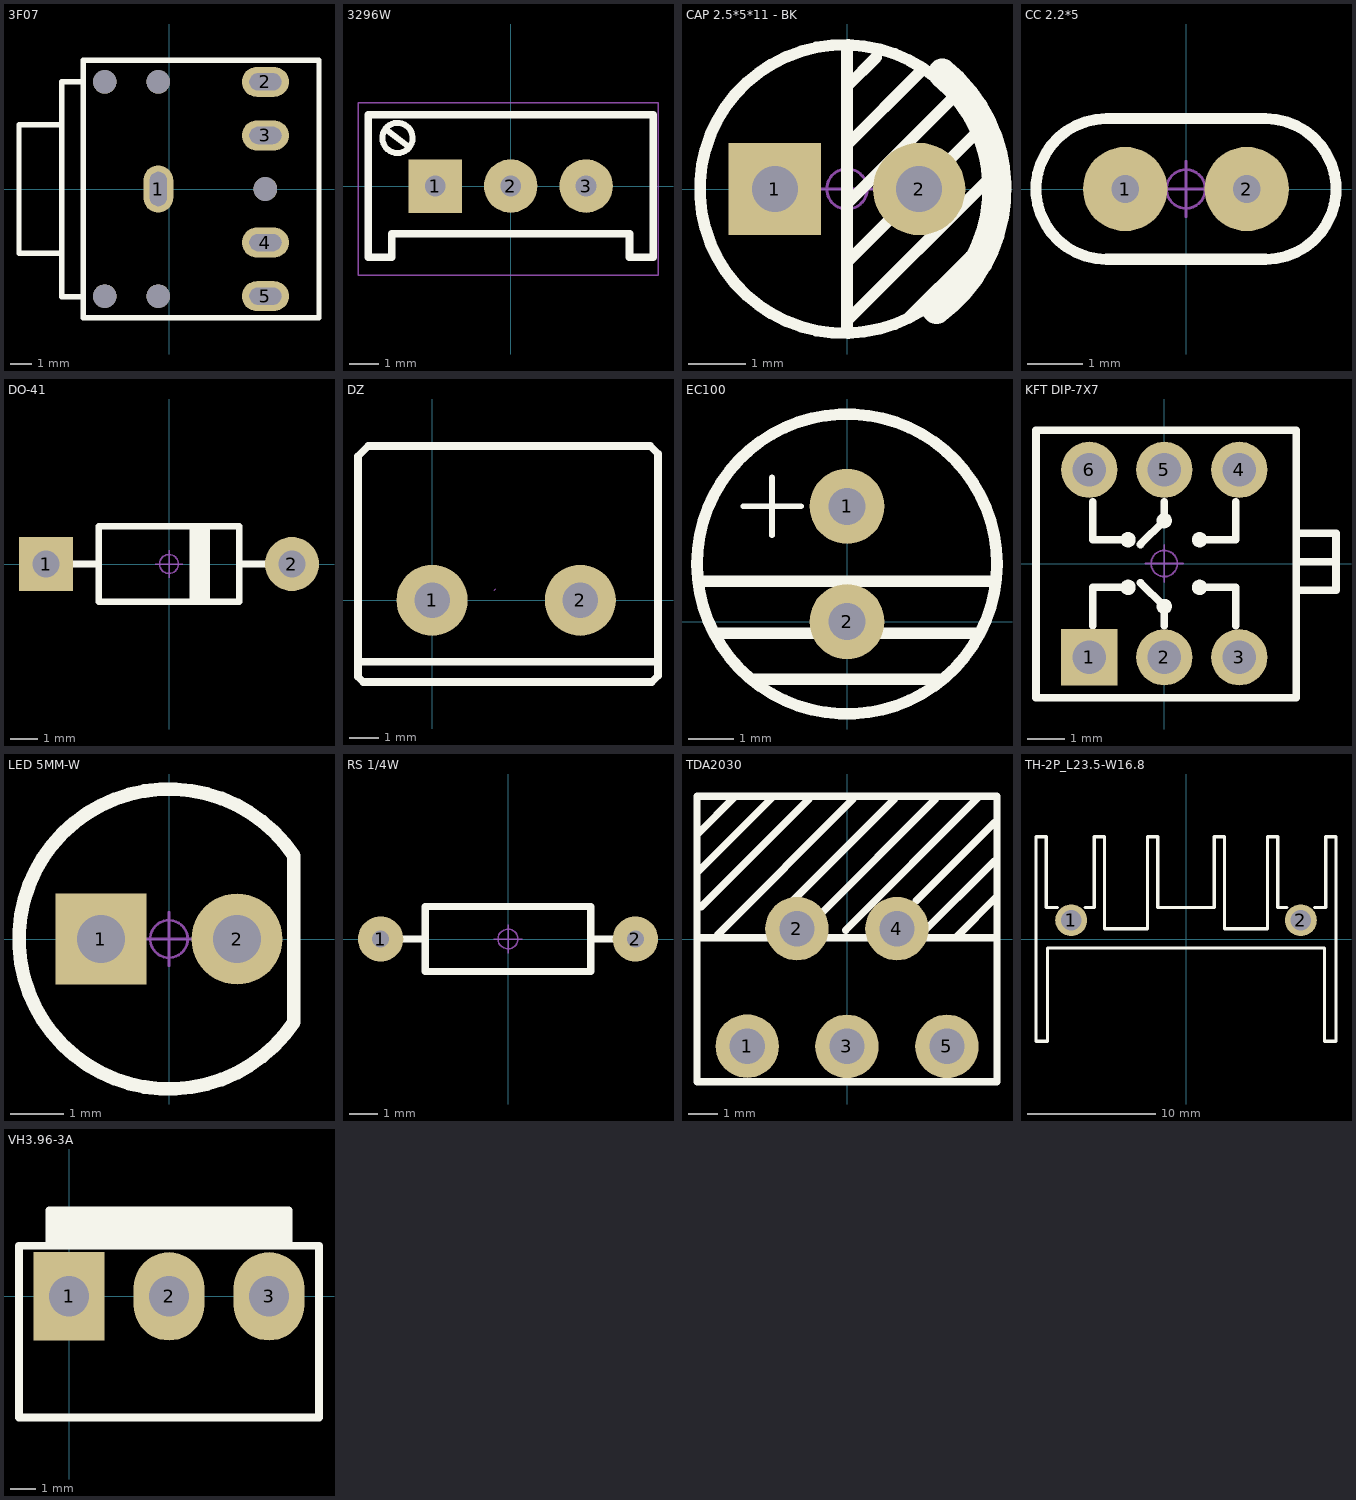
[diagram p0: the footprints below, top view; thin cyan lines are the x and y axes]
# Altium footprint library MISC82779.PcbLib: 13 footprints
Each footprint in its own frame and in the unit in brackets; x right, y up, seen from the top. Pads: shape width x height; smd on the part's side, far side on the other; paste and mask are expansions set on the pad; w line width, h text height; cw(c..) or ccw(c..) is an arc to the next point about the centre after c.

## 3F07 [mm]
pads (10):
  oval 1.4x2.2 hole 0.8 slot 1.6 at 90 deg paste+0 mask+0.051: 1(-0.5,0)
  oval 2.2x1.4 hole 0.8 slot 1.5 at 0 deg paste+0 mask+0.051: 2(4.5,5) 3(4.5,2.5) 4(4.5,-2.5) 5(4.5,-5)
  round 1.1 hole 1.1 unplated paste+0: ""(-3,-5) ""(-3,5) ""(-0.5,-5) ""(-0.5,5) ""(4.5,0)
Top Overlay:
  lines w0.254: -5,-3 -7,-3 -7,3 -5,3 ; -4,-5.026 -5,-5.026 -5,5 -4,5 ; -4,5 -4,6 7,6 7,-6 -4,-6 -4,-5 -4,5
Mechanical 15:
  circle w0.45: c4.5,0 r0.225
  circle w0.45: c-3,5 r0.225
  circle w0.45: c-0.5,5 r0.225
  circle w0.45: c-0.5,-5 r0.225
  circle w0.45: c-3,-5 r0.225

## 3296W [mm]
pads (3):
  rect 1.8x1.8 hole 0.7: 1(-2.54,0)
  round 1.8 hole 0.7: 2(0,0) 3(2.54,0)
Top Overlay:
  lines w0.2: -3.302,1.651 ccw(c-3.81,1.618) -3.301,1.608
  lines w0.203: -4.2,1.9 -3.464,1.348
  lines w0.254: -4.8,-2.4 -4.8,2.4 4.8,2.4 4.8,-2.4 4,-2.4 4,-1.6 -4,-1.6 -4,-2.4 -4.8,-2.4
Mechanical 15:
  lines w0.05: -5.14,-3 4.96,-3 4.96,2.8 -5.14,2.8 -5.14,-3
3D body "3296.STEP": height 11.52, standoff -3.48, extent -4.75,-2.4 4.75,2.4

## CAP 2.5*5*11 - BK [mm]
pads (2):
  rect 1.6x1.6 hole 0.8: 1(-1.25,0)
  round 1.6 hole 0.8: 2(1.25,0)
Top Overlay:
  circle w0.2: c-0.05,0 r2.5
  lines w0.2: 0,-2.489 0,2.413 ; 0,-2.286 2.438,0.152 ; 0,-1.27 2.222,0.953 ; 0,-0.254 1.841,1.587 ; 0,0.762 1.27,2.032 ; 0,1.778 0.508,2.286 ; 1.079,-2.222 2.134,-1.168
  lines w0.5: 1.552,-2.086 ccw(c0,0) 1.651,2.008
Mechanical 15:
  circle w0.05: c0,0 r0.35
  lines w0.05: -0.5,0 0.5,0 ; 0,-0.5 0,0.5
3D body "CAP 2.5X5X11.STEP": height 11.04, standoff -3.42, extent -2.5,-2.499 2.51,2.499

## CC 2.2*5 [mm]
pads (2):
  round 1.524 hole 0.5: 1(-1.1,0) 2(1.1,0)
Top Overlay:
  lines w0.2: -1.44,-1.271 cw(c-1.44,0) -1.44,1.271 1.44,1.271 cw(c1.44,0) 1.44,-1.271 -1.44,-1.269
Mechanical 15:
  circle w0.05: c0,0 r0.35
  lines w0.05: -0.5,0 0.5,0 ; 0,-0.5 0,0.5
3D body "CC 2.2X5.STEP": height 4.8, standoff -3.5, extent -2.4,-0.917 2.4,0.918

## DO-41 [mm]
pads (2):
  rect 2x2 hole 1: 1(-4.55,0)
  round 2 hole 1: 2(4.55,0)
Top Overlay:
  rectangle: 0.762,-1.397 1.524,1.397
  lines w0.254: -3.556,0 -2.6,0 ; 2.6,0 3.556,0 ; -2.6,-1.397 -2.6,1.397 2.6,1.397 2.6,-1.397 -2.6,-1.397
Mechanical 15:
  circle w0.05: c0,0 r0.35
  lines w0.05: -0.5,0 0.5,0 ; 0,-0.5 0,0.5
3D body "DO-41.STEP": height 2.65, standoff -3.45, extent -4.925,-1.288 4.975,1.314

## DZ [mm]
pads (2):
  round 2.4 hole 1.2: 1(0,0) 2(5,0)
Top Overlay:
  lines w0.254: -2.5,-2.073 7.5,-2.073 ; -2.5,-2.58 -2.326,-2.754 7.406,-2.754 7.62,-2.54 7.62,4.953 7.366,5.207 -2.159,5.207 -2.5,4.866 -2.5,-2.58
Mechanical 15:
  lines w0.003: 2.094,0.341 2.144,0.392

## EC100 [mil]
pads (2):
  round 65 hole 32: 1(0,100) 2(0,0)
Top Overlay:
  circle w10: c0,50 r130.1
  lines w5: -90,100 -40,100 ; -65,75 -65,125
  lines w10: -125,35 125,35 ; -115,-10 115,-10 ; -80,-50 80,-50

## KFT DIP-7X7 [mm]
pads (6):
  rect 1.5x1.5 hole 0.9: 1(-2,-2.5)
  round 1.5 hole 0.9: 2(0,-2.5) 3(2,-2.5) 4(2,2.5) 5(0,2.5) 6(-2,2.5)
Top Overlay:
  circle w0.254: c0.94,-0.635 r0.076
  circle w0.254: c-0.965,-0.635 r0.076
  circle w0.254: c0,-1.143 r0.076
  circle w0.254: c0,1.143 r0.076
  circle w0.254: c-0.965,0.635 r0.076
  circle w0.254: c0.94,0.635 r0.076
  lines w0.203: -1.905,-1.651 -1.905,-0.635 -0.889,-0.635 ; -1.905,1.651 -1.905,0.635 -0.889,0.635 ; -0.635,-0.508 0,-1.143 0,-1.651 ; -0.635,0.508 0,1.143 0,1.651 ; 1.016,-0.635 1.905,-0.635 1.905,-1.651 ; 1.016,0.635 1.905,0.635 1.905,1.651 ; 3.514,0.05 4.579,0.05 ; 3.563,-0.712 4.579,-0.712 4.579,0.812 3.563,0.812 ; -3.42,-3.581 3.514,-3.581 3.514,2.54 3.514,3.556 -3.42,3.556 -3.42,-3.581
Mechanical 15:
  circle w0.05: c0,0 r0.35
  lines w0.05: -0.5,0 0.5,0 ; 0,-0.5 0,0.5
3D body "SLSW 7x7.STEP": height 11.2, standoff -3.2, extent -3.5,-3.5 3.5,3.5

## LED 5MM-W [mm]
pads (2):
  rect 1.7x1.7 hole 0.9: 1(-1.27,0)
  round 1.7 hole 0.9: 2(1.27,0)
Top Overlay:
  lines w0.254: 2.33,-1.553 cw(c0,0) 2.33,1.553 2.33,-1.553
Mechanical 15:
  circle w0.05: c0,0 r0.35
  lines w0.05: -0.5,0 0.5,0 ; 0,-0.5 0,0.5
3D body "LED 5mm-W.STEP": height 4.5, standoff -3.45, extent -1.983,-0.795 2.076,0.805
3D body "LED 5mm玻璃罩.STEP": height 8.75, standoff 0.05, extent -2.85,-2.85 2.454,2.85

## RS 1/4W [mm]
pads (2):
  round 1.6 hole 0.6: 1(-4.5,0) 2(4.5,0)
Top Overlay:
  lines w0.254: -3.683,0 -3.048,0 ; 3.048,0 3.683,0 ; -2.921,-1.143 -2.921,1.143 2.921,1.143 2.921,-1.143 -2.921,-1.143
Mechanical 15:
  circle w0.05: c0,0 r0.35
  lines w0.05: -0.5,0 0.5,0 ; 0,-0.5 0,0.5
3D body "RS 1-4W.STEP": height 2.32, standoff -3.49, extent -4.725,-1.16 4.725,1.16

## TDA2030 [mm]
pads (5):
  round 2.159 hole 1.2 paste+0 mask+0.051: 1(-3.392,-3.644) 2(-1.7,0.35) 3(0,-3.65) 4(1.7,0.35) 5(3.4,-3.65)
Top Overlay:
  lines w0.254: -5.05,2.3 -2.55,4.8 ; -5.05,3.6 -3.85,4.8 ; -4.95,1.1 -1.3,4.75 ; -4.4,0.15 0.2,4.75 ; -1.95,1.2 1.6,4.75 ; -0.95,0.8 3,4.75 ; -0.05,0.3 4.45,4.8 ; 2.35,1.3 5,3.95 ; 2.5,0.15 5,2.65 ; 3.75,0.1 5.05,1.4 ; -5.1,0.05 5.1,0.05 ; -5.1,0.05 -5.1,-4.85 5.1,-4.85 5.1,0.05 ; -5.1,0.05 5.1,0.05 ; -5.1,0.05 -5.1,4.85 5.1,4.85 5.1,0.05

## TH-2P_L23.5-W16.8 [mm]
pads (2):
  round 2.5 hole 1.6 paste+0 mask+0.05: 1(-8.999,1.47) 2(9.001,1.47)
Top Overlay:
  lines w0.254: -10.091,2.47 -10.949,2.47 -10.949,2.97 -10.949,8 -11.749,8 -11.749,-8 -10.849,-8 -10.85,-7.863 -10.85,-2.17 -10.85,-0.7 10.85,-0.7 10.85,-2.17 10.85,-7.863 10.849,-8 11.749,-8 11.749,8 10.951,8 10.951,2.471 10.093,2.47 ; -7.907,2.47 -7.179,2.47 -7.179,8 -6.779,8 -6.379,8 -6.379,2.47 -6.379,0.8 -3.009,0.8 -3.009,2.47 -3.009,8 -2.609,8 -2.209,8 -2.209,2.47 2.211,2.47 2.211,8 2.611,8 3.011,8 3.011,2.47 3.011,0.8 6.381,0.8 6.381,2.47 6.381,8 6.781,8 7.181,8 7.181,2.47 7.909,2.47
Mechanical 15:
  circle w0.3: c-8.399,1.07 r0.15

## VH3.96-3A [mm]
pads (3):
  rect 2.8x3.5 hole 1.6: 1(0,0)
  oval 2.8x3.5 hole 1.6: 2(3.96,0) 3(7.92,0)
Top Overlay:
  lines w0.3: -0.78,2 -0.78,3.4 8.7,3.4 8.7,2 ; -0.78,2.286 8.7,2.286 ; -0.78,2.413 8.7,2.413 ; -0.78,2.667 8.7,2.667 ; -0.78,2.921 8.7,2.921 ; -0.78,3.175 8.7,3.175 ; -1.98,-4.8 -1.98,2 9.9,2 9.9,-4.8 -1.98,-4.8
3D body "VH3.96-3A.STEP": height 14.6, standoff -3.6, extent -1.98,-4.8 9.9,3.6